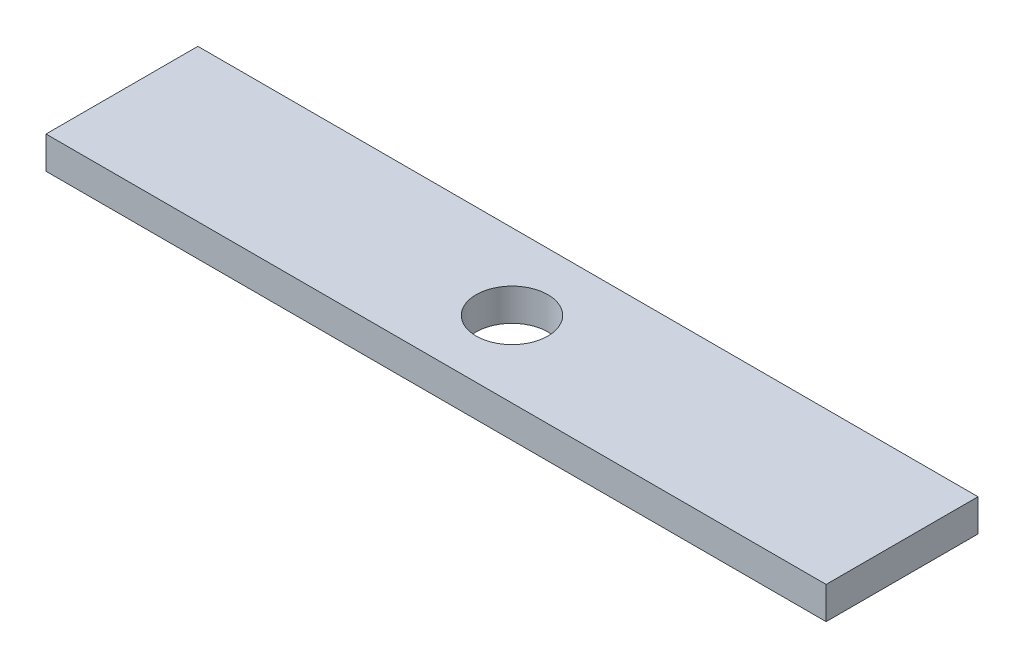
SolidWorks part; units mm, degrees
ref_plane "Front Plane" through (0, 0, 0) normal (0, 0, 1) x (1, 0, 0)
ref_plane "Top Plane" through (0, 0, 0) normal (0, 1, 0) x (1, 0, 0)
ref_plane "Right Plane" through (0, 0, 0) normal (1, 0, 0) x (0, 0, -1)
sketch "Sketch1" plane through (0, 0, 0) normal (0, 1, 0) x (1, 0, 0)
  line L1 (0, 0) -> (108.7323, 0)
  line L2 (0, 0) -> (0, 21.1681)
  line L3 (0, 21.1681) -> (108.7323, 21.1681)
  line L4 (108.7323, 0) -> (108.7323, 21.1681)
  circle A1 centre (54.3661, 10.584) radius 5
extrude "Boss-Extrude1" add sketch "Sketch1" along normal blind 4.5
